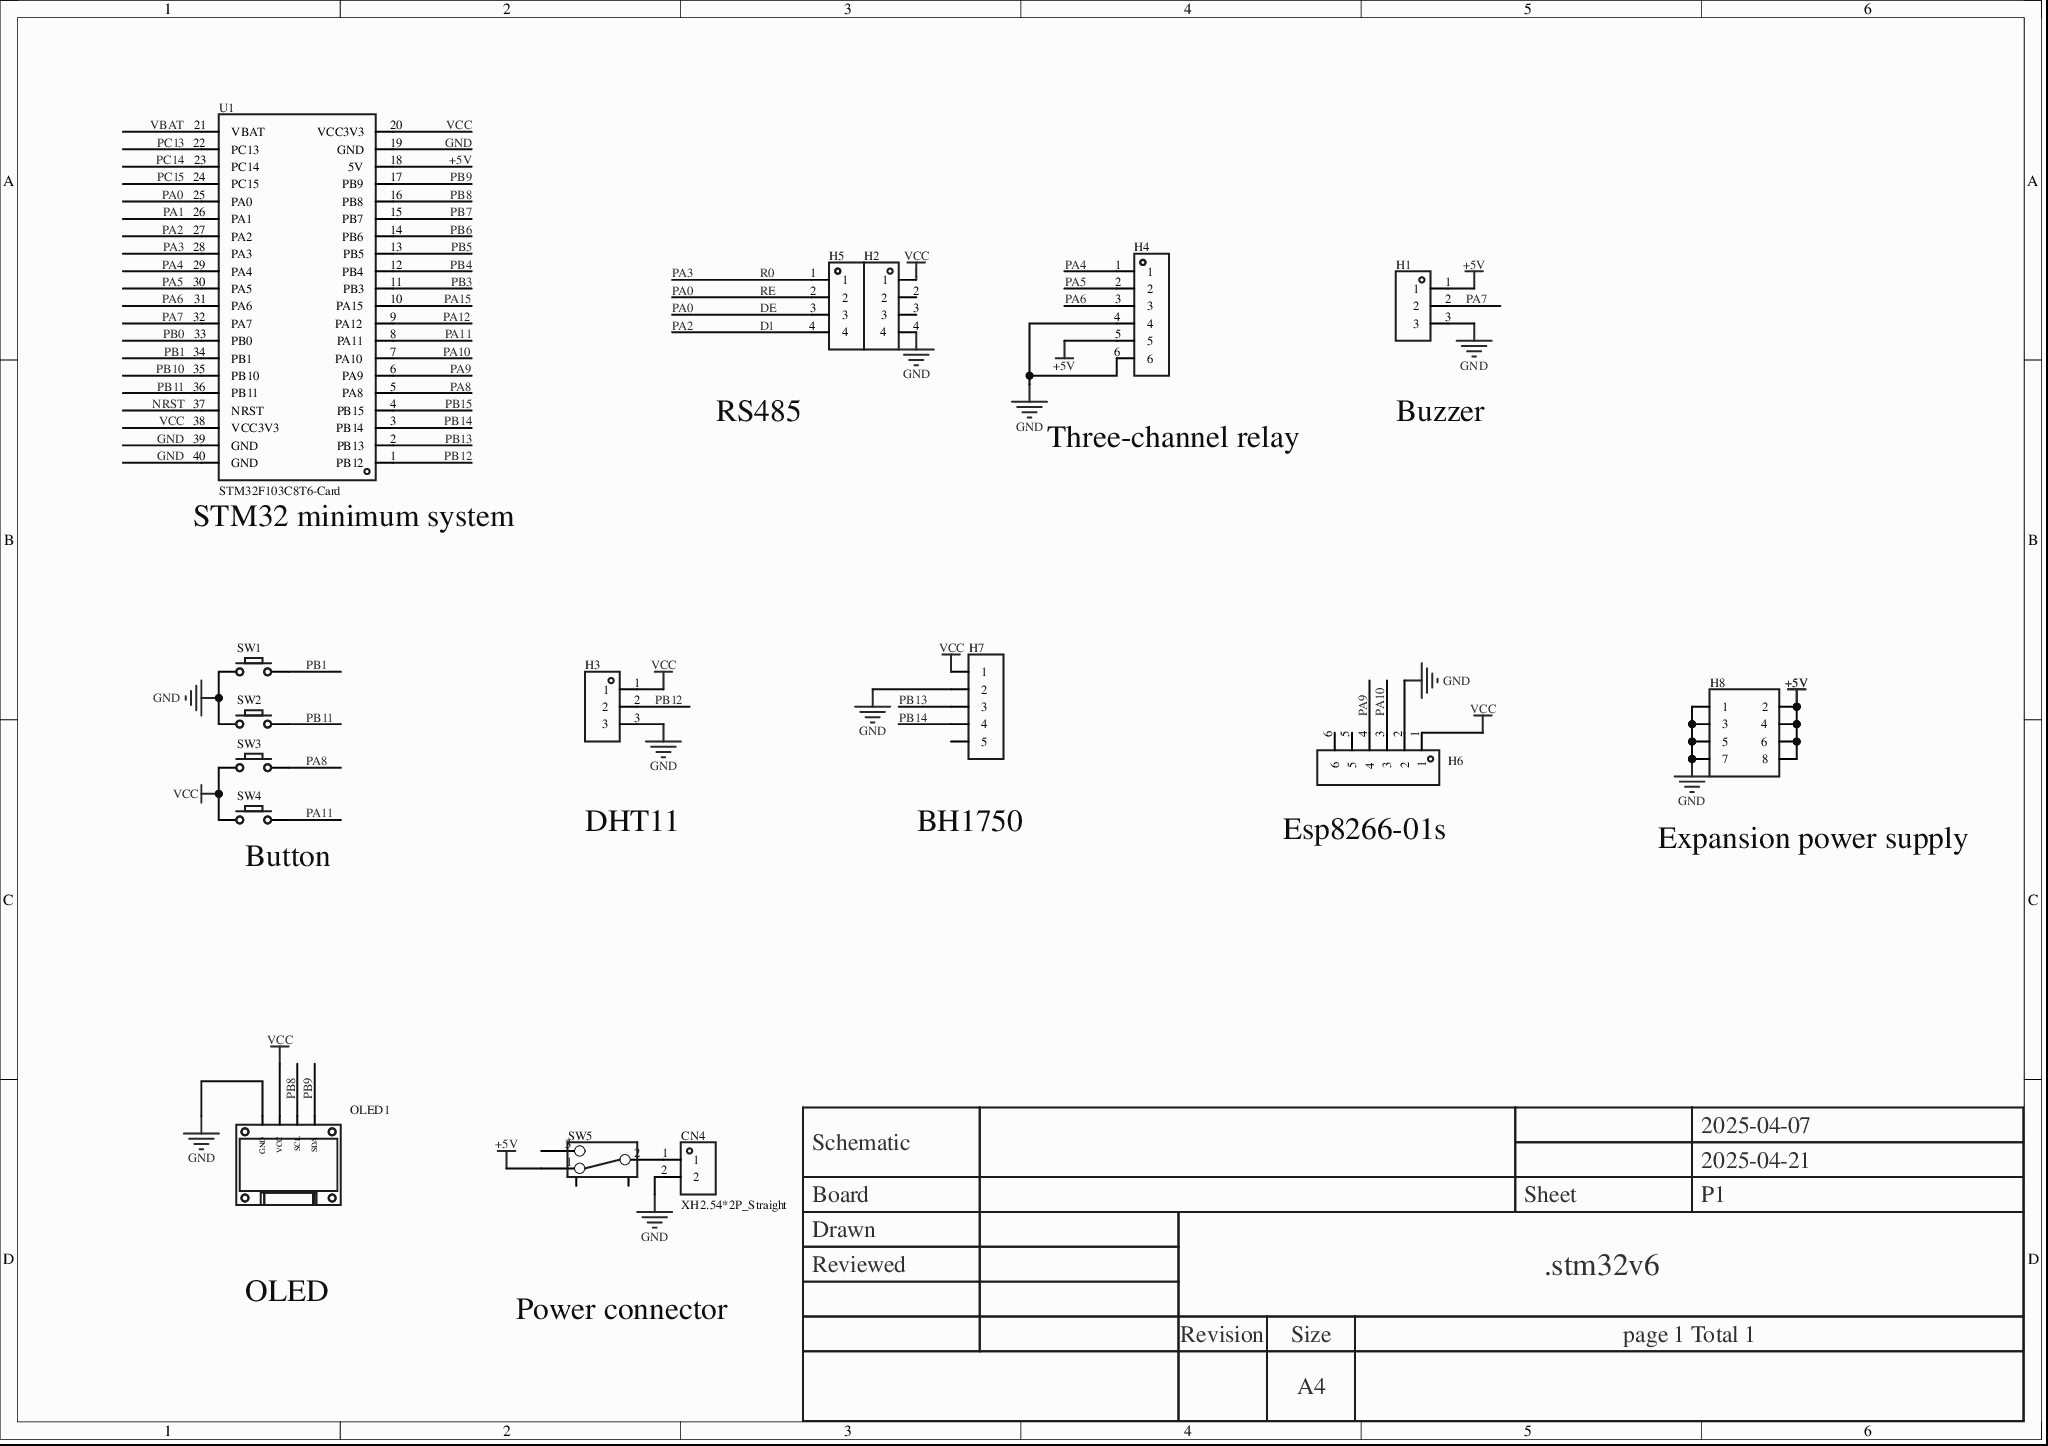
[diagram p0: MISC89004-3.schdoc]
# Altium project MISC89004-2.PrjPcb
1 sheet, 16 parts. Net scope: global (net labels, ports and power ports of the same name join across sheets).
Board file: MISC89004.pcbdoc

## Sheet MISC89004-3.schdoc
size 297 x 209 mm; Version: V1.0; @Project Name: MISC89004; @Page Count: 1; @Update Date: 2026-04-13; @Create Date: 2026-04-13; @Schematic Name: MISC89004; @Page No: 1; @Create Time: 23:22:16; @Update Time: 17:32:40; @Board Name: MISC89004

### Parts
CN4  XH2.54*2P_Straight  [CONN-TH_2P-P2.50-XH2.54-2P]
H1  (no value)  [HDR-TH_3P-P2.54-V-F]
H2  (no value)  [HDR-TH_4P-P2.54-V-F]
H3  (no value)  [HDR-TH_3P-P2.54-V-F]
H4  (no value)  [HDR-TH_6P-P2.54-V-F]
H5  (no value)  [HDR-TH_4P-P2.54-V-F]
H6  (no value)  [HDR-TH_6P-P2.54-V-F]
H7  (no value)  [HDR-TH_5P-P2.54-V-F]
H8  (no value)  [HDR-TH_8P-P2.54-V-F-R2-C4-S2.54-1]
OLED1  (no value)  [0.96OLED_4P]
SW1  (no value)  [Key_TH_3.5x6x4.3]
SW2  (no value)  [Key_TH_3.5x6x4.3]
SW3  (no value)  [Key_TH_3.5x6x4.3]
SW4  (no value)  [Key_TH_3.5x6x4.3]
SW5  (no value)  [拨动开关]
U1  STM32F103C8T6-Card  [CONN-TH_L53.3-W22.9_STM32F103C8T6-CARD]

### Nets
+5V: H1.1 H4.5 H8.2 H8.4 H8.6 H8.8 SW5.1 U1.18(5V)
GND: CN4.2 H1.3 H2.4 H3.3 H4.4 H4.6 H6.2 H7.2 H8.1 H8.3 H8.5 H8.7 OLED1.1(GND) SW1.A SW2.A U1.19(GND) U1.39(GND) U1.40(GND)
VCC: H2.1 H3.1 H6.1 H7.1 OLED1.2(VCC) SW3.A SW4.A U1.20(VCC3V3) U1.38(VCC3V3)
D1: H5.4 U1.27(PA2)  [also labelled PA2]
DE: H5.2 H5.3 U1.25(PA0)  [also labelled PA0, RE]
NRST: U1.37(NRST)
PA1: U1.26(PA1)
PA3: H5.1 U1.28(PA3)  [also labelled R0]
PA4: H4.1 U1.29(PA4)
PA5: H4.2 U1.30(PA5)
PA6: H4.3 U1.31(PA6)
PA7: H1.2 U1.32(PA7)
PA8: SW3.B U1.5(PA8)
PA9: H6.4 U1.6(PA9)
PA10: H6.3 U1.7(PA10)
PA11: SW4.B U1.8(PA11)
PA12: U1.9(PA12)
PA15: U1.10(PA15)
PB0: U1.33(PB0)
PB1: SW1.B U1.34(PB1)
PB3: U1.11(PB3)
PB4: U1.12(PB4)
PB5: U1.13(PB5)
PB6: U1.14(PB6)
PB7: U1.15(PB7)
PB8: OLED1.3(SCL) U1.16(PB8)
PB9: OLED1.4(SDA) U1.17(PB9)
PB10: U1.35(PB10)
PB11: SW2.B U1.36(PB11)
PB12: H3.2 U1.1(PB12)
PB13: H7.3 U1.2(PB13)
PB14: H7.4 U1.3(PB14)
PB15: U1.4(PB15)
PC13: U1.22(PC13)
PC14: U1.23(PC14)
PC15: U1.24(PC15)
VBAT: U1.21(VBAT)
NetCN4_1: CN4.1 SW5.2

Not connected (* = marked no-connect by the designer): H2 2 3; H6 5 6; H7 5; SW5 3 4 5

### Notes on the sheet
- RS485
- Buzzer
- (near H4) Three-channel relay
- (near U1) STM32 minimum system
- (near SW4) Button
- DHT11
- (near H7) BH1750
- (near H6) Esp8266-01s
- (near H8) Expansion power supply
- OLED
- Power connector
- 2025-04-07
- Schematic
- Board
- Sheet
- 2025-04-21
- P1
- Drawn
- Reviewed
- .stm32v6
- Revision
- Size
- A4
- page 1 Total 1

### Library data of the parts
CN4 = XH2.54*2P_直插: 3D Model: 325c595e30db4df8abe76612dd40b0fa0819f05c4eef4c71ace90d822a990e87; 3D Model Transform: 295.275,228.346,0,180,0,0,-0.002,-20.079,-137.795; AddInBom: yes; Device: XH2.54*2P_Straight; Symbol: XH2.54*2P_Straight; LCSC Part Name: XH2.54*2P_直插; Supplier Part: C9900008615; Manufacturer Part: XH2.54*2P_直插; Supplier Footprint: XH2.54_2P; JLCPCB Part Class: Extended Part; Supplier: LCSC; FootprintName: CONN-TH_2P-P2.50-XH2.54-2P; ConvertToPcb: yes; ModelName: CONN-TH_2P-P2.50-XH2.54-2P
H1 H3 = HDR-F_2.54_1x3P: Symbol: PM254V-11-03-H85; 3D Model: f3b3cc5aae9641bf9e56fc160cef875b; 3D Model Transform: 299.9994,100,0,0,0,0,0,0,-118.11; ConvertToPcb: yes; ModelName: HDR2.54-F-LI-1X3P; Device: HDR-F_2.54_1x3P; Supplier Part: C541850; Supplier Footprint: 插件; FootprintName: HDR-TH_3P-P2.54-V-F; AddInBom: yes
H2 H5 = HDR-F_2.54_1x4P: Symbol: 2.54-1*4P female; 3D Model: d187812051054f85879fcaa51a310d8e0819f05c4eef4c71ace90d822a990e87; 3D Model Transform: 419.6842,98.464,0,0,0,0,0,0,-118.11; ConvertToPcb: yes; Device: HDR-F_2.54_1x4P; Supplier Part: C2718488; Supplier Footprint: 插件; AddInBom: yes; FootprintName: HDR-TH_4P-P2.54-V-F; ModelName: HDR-TH_4P-P2.54-V-F
H4 H6 = HDR-F_2.54_1x6P: Symbol: Header-Female-2.54_1x6; ConvertToPcb: yes; ModelId: 0f5bcf94dcda47d085f24cdca1696fe9; ModelTransform: 619.684,94.488,0,0,0,0,0,0,-125.984; Device: HDR-F_2.54_1x6P; AddInBom: yes; SupplierPart: C40877; Supplier Footprint: 插件; FootprintName: HDR-TH_6P-P2.54-V-F; ModelName: HDR-TH_6P-P2.54-V-F
H7 = HDR-F_2.54_1x5P: Symbol: Header-Female-2.54_1x5; ConvertToPcb: yes; ModelId: f49cb6116a3d45e5a64915bf3e00773f; ModelTransform: 519.684,98.464,0,0,0,0,0,0,-124.016; Device: HDR-F_2.54_1x5P; AddInBom: yes; SupplierPart: C50950; Supplier Footprint: 插件; FootprintName: HDR-TH_5P-P2.54-V-F; ModelName: HDR-TH_5P-P2.54-V-F
H8 = HDR-F_2.54_2x4: Symbol: HDR-F-2.54_2x4; ConvertToPcb: yes; ModelId: 64729f32a5874cf59655d275a66f10500819f05c4eef4c71ace90d822a990e87; ModelName: HDR2.54-F-LI-2X4P; ModelTransform: 399.999,200,0,0,0,0,0,0,-118.11; Device: HDR-F_2.54_2x4; AddInBom: yes; SupplierPart: C92271; Supplier Footprint: 插件; FootprintName: HDR-TH_8P-P2.54-V-F-R2-C4-S2.54-1
OLED1 = 0.96OLED模块_4P: Device: 0.96OLED module_4P; ConvertToPcb: yes; ModelId: 79c000fdb68d45a296c2e9bedf4f9055; ModelTransform: 1393.69792,1318.895,0,0,0,0,0,-560.079,-137.795; Symbol: 0.96OLED module_4P; FootprintName: 0.96OLED_4P; AddInBom: yes; Supplier Footprint: 插件; ModelName: 0.96OLED_4P
SW1-SW4 = Key_TH_3.5x6x4.3: ConvertToPcb: yes; ModelId: c3523f9014d949d7ba5445190a3178990819f05c4eef4c71ace90d822a990e87; ModelName: SW-TH_L6.0-W3.5-H5.0-P6.5; ModelTransform: 308.49,137.8,335.08,0,0,0,0,0,-129.92; Symbol: Key_TH_3.5x6x4.3; Device: Key_TH_3.5x6x4.3; AddInBom: yes; Supplier Footprint: 插件; FootprintName: Key_TH_3.5x6x4.3
SW5 = 拨动开关_正: Device: Toggle switch_upright; Symbol: Toggle switch; ConvertToPcb: yes; ModelId: 4321fe59a4074cbfb4989553f297c68f0819f05c4eef4c71ace90d822a990e87; ModelName: SW-TH_SS-12D02-VG4; ModelTransform: 370.09,208.7,472.35,0,0,0,0,0,-110; FootprintName: Toggle switch; AddInBom: yes; Supplier Footprint: 插件
U1 = STM32F103C8T6-Card: AddInBom: yes; Device: STM32F103C8T6-Card; Symbol: STM32F103C8T6-CARD; FootprintName: CONN-TH_L53.3-W22.9_STM32F103C8T6-CARD; LCSC Part Name: STM32F103C8T6-Card; SupplierPart: C9900077949; ManufacturerPart: STM32F103C8T6-Card; Supplier Footprint: 插件; Supplier: LCSC; ConvertToPcb: yes